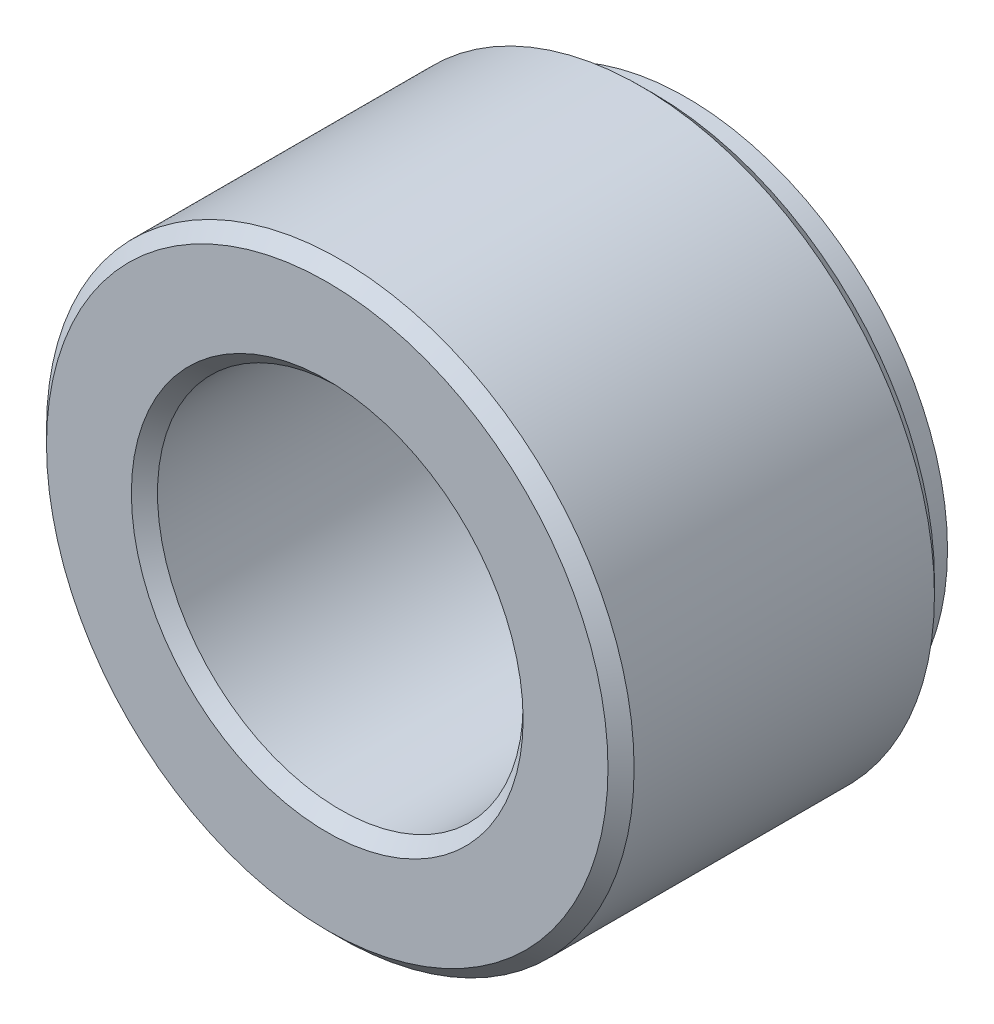
from build123d import *

# Parameters (mm, degrees)
SKETCH8_R                  = 22.5
BOSS_EXTRUDE2_DEPTH        = 25
M30X2_0_TAPPED_HOLE1_D     = 28
M30X2_0_TAPPED_HOLE1_DEPTH = 70
M30X2_0_TAPPED_HOLE1_TIP   = 8.412048666
BOSS_EXTRUDE3_START        = 2.5
SKETCH11_R                 = 20
SKETCH11_R_2               = 14
BOSS_EXTRUDE3_DEPTH        = 2.5
CHAMFER1_SIZE              = 1


with BuildPart() as part:
    # Sketch8 → Boss-Extrude2 (new body)
    with BuildSketch(Plane.XY):
        with Locations((-69.420997024, 0)):
            Circle(SKETCH8_R)
    extrude(amount=BOSS_EXTRUDE2_DEPTH)

    # M30x2.0 Tapped Hole1
    with Locations(Plane(origin=(-69.420997024, 0, 25), x_dir=(1, 0, 0), z_dir=(0, 0, 1))):
        with Locations((0, 0)):
            Hole(M30X2_0_TAPPED_HOLE1_D / 2, depth=M30X2_0_TAPPED_HOLE1_DEPTH)
            with Locations((0, 0, -(M30X2_0_TAPPED_HOLE1_DEPTH + M30X2_0_TAPPED_HOLE1_TIP / 2))):  # 118° drill point
                Cone(0, M30X2_0_TAPPED_HOLE1_D / 2, M30X2_0_TAPPED_HOLE1_TIP, mode=Mode.SUBTRACT)

    # Sketch11 → Boss-Extrude3 (add)
    with BuildSketch(Plane(origin=(0, 0, 0), x_dir=(-1, 0, 0), z_dir=(0, 0, -1)).offset(BOSS_EXTRUDE3_START)):
        with Locations(Location((69.420997024, 0, 0), (0, 0, 180))):
            Circle(SKETCH11_R)
        with Locations(Location((69.420997024, 0, 0), (0, 0, 180))):
            Circle(SKETCH11_R_2, mode=Mode.SUBTRACT)
    extrude(amount=-BOSS_EXTRUDE3_DEPTH)

    # Chamfer1
    chamfer1_edges = [part.edges().sort_by_distance(p)[0] for p in [
        (-91.920997024, 0, 0),
        (-91.920997024, 0, 25),
        (-55.420997024, 0, 25),
    ]]
    chamfer(chamfer1_edges, length=CHAMFER1_SIZE)


solid = part.part
